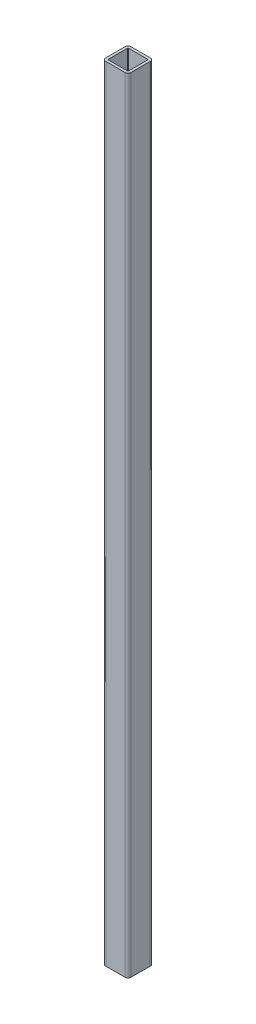
from build123d import *

# Parameters (mm, degrees)
EXTRUDE_1_DEPTH = 1550


with BuildPart() as part:
    # 草图1 → 凸台-拉伸1 (new body)
    with BuildSketch(Plane(origin=(0, 0, 0), x_dir=(1, 0, 0), z_dir=(0, 1, 0))):
        with BuildLine():
            Line((-19, -12.278106509), (19, -12.278106509))
            ThreePointArc((19, -12.278106509), (23.242640687, -10.520747196), (25, -6.278106509))
            Line((25, -6.278106509), (25, 31.721893491))
            ThreePointArc((25, 31.721893491), (23.242640687, 35.964534178), (19, 37.721893491))
            Line((19, 37.721893491), (-19, 37.721893491))
            ThreePointArc((-19, 37.721893491), (-23.242640687, 35.964534178), (-25, 31.721893491))
            Line((-25, 31.721893491), (-25, -6.278106509))
            ThreePointArc((-25, -6.278106509), (-23.242640687, -10.520747196), (-19, -12.278106509))
        make_face()
        with BuildLine():
            Line((-19, -7.278106509), (19, -7.278106509))
            ThreePointArc((19, -7.278106509), (19.707106781, -6.98521329), (20, -6.278106509))
            Line((20, -6.278106509), (20, 31.721893491))
            ThreePointArc((20, 31.721893491), (19.707106781, 32.429000272), (19, 32.721893491))
            Line((19, 32.721893491), (-19, 32.721893491))
            ThreePointArc((-19, 32.721893491), (-19.707106781, 32.429000272), (-20, 31.721893491))
            Line((-20, 31.721893491), (-20, -6.278106509))
            ThreePointArc((-20, -6.278106509), (-19.707106781, -6.98521329), (-19, -7.278106509))
        make_face(mode=Mode.SUBTRACT)
    extrude(amount=EXTRUDE_1_DEPTH)


solid = part.part
